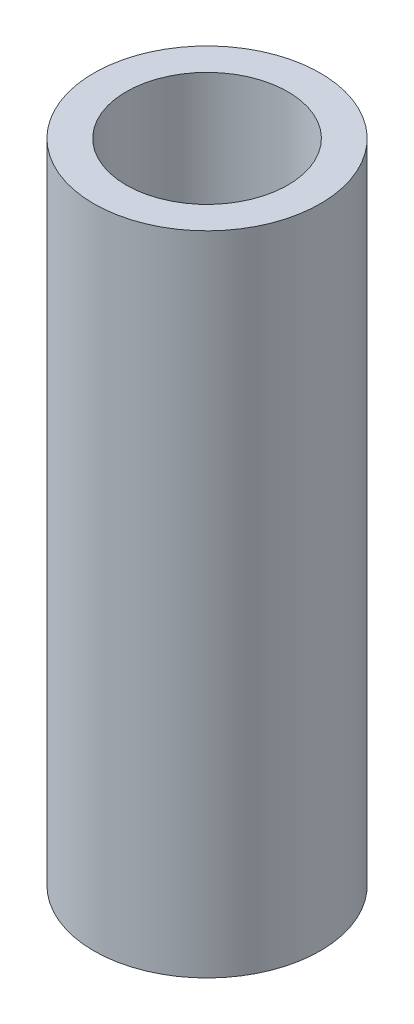
from build123d import *

# Parameters (mm, degrees)
SKETCH1_R           = 17.5
SKETCH1_R_2         = 12.5
BOSS_EXTRUDE1_DEPTH = 100
FILLET1_R           = 2


with BuildPart() as part:
    # Sketch1 → Boss-Extrude1 (new body)
    with BuildSketch(Plane(origin=(0, 0, 0), x_dir=(1, 0, 0), z_dir=(0, 1, 0))):
        with Locations(Location((0, 0, 0), (0, 0, 270))):
            Circle(SKETCH1_R)
        with Locations(Location((0, 0, 0), (0, 0, 270))):
            Circle(SKETCH1_R_2, mode=Mode.SUBTRACT)
    extrude(amount=BOSS_EXTRUDE1_DEPTH)

    # Fillet1
    fillet1_edges = [part.edges().sort_by_distance(p)[0] for p in [
        (0, 0, -12.5),
    ]]
    fillet(fillet1_edges, radius=FILLET1_R)


solid = part.part
